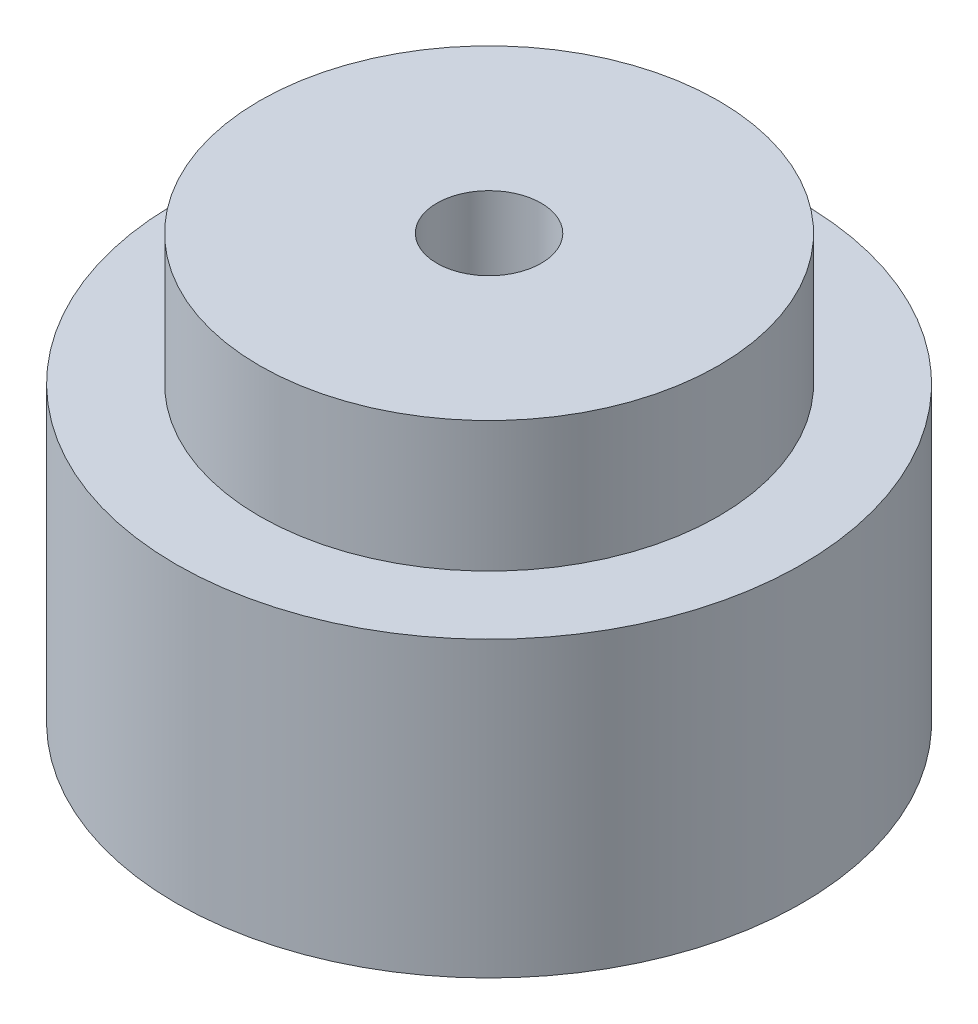
from build123d import *


with BuildPart() as part:
    # 草图1 → 旋转1 (revolve)
    with BuildSketch(Plane.XY, mode=Mode.PRIVATE) as revolve_1_sk:
        Polygon((-4, 32.5), (-17.6, 32.5), (-17.6, 22.5), (-24, 22.5), (-24, 0), (-20, 0), (-20, 15), (-4, 20.6), align=None)
    revolve(revolve_1_sk.sketch.rotate(Axis((0, 61.8, 0), (0, -1, 0)), 270), axis=Axis((0, 61.8, 0), (0, -1, 0)))


solid = part.part
